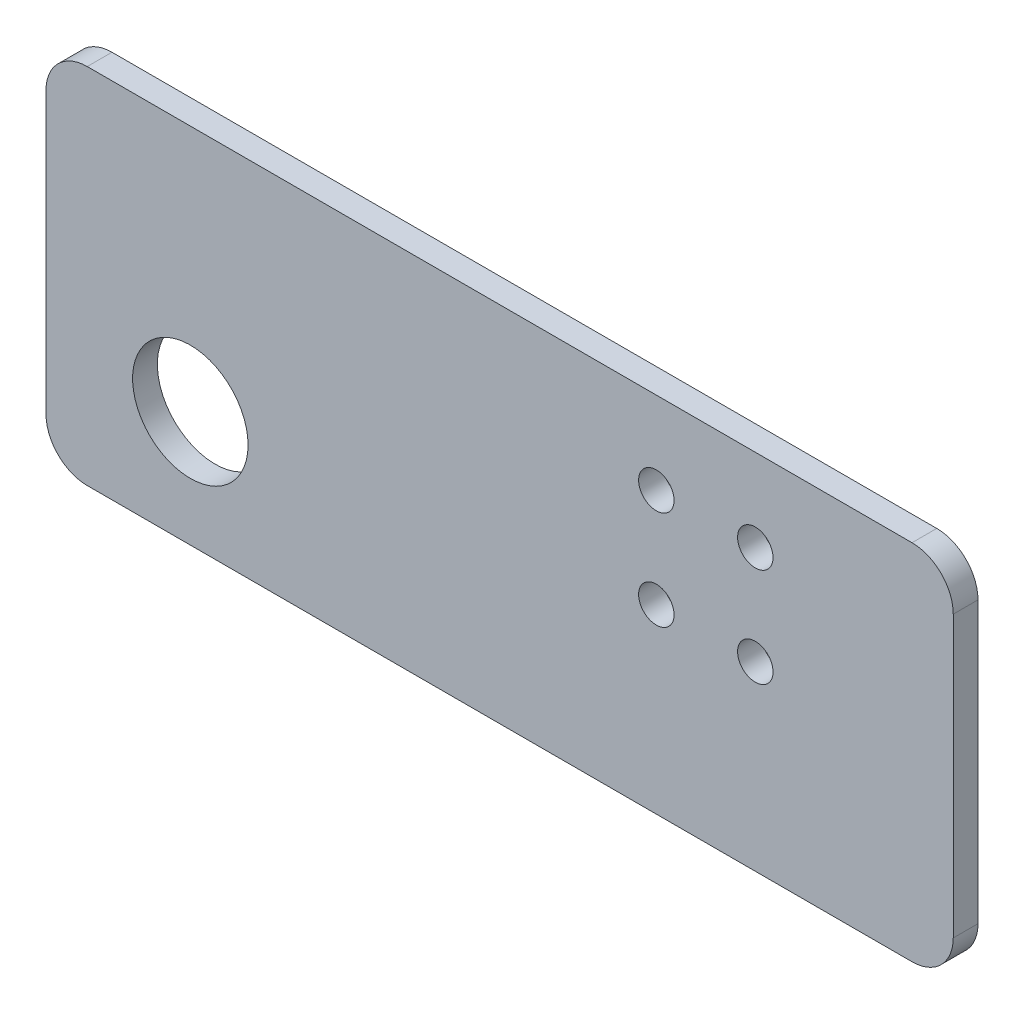
SolidWorks part; units mm, degrees
ref_plane "前视基准面" through (0, 0, 0) normal (0, 0, 1) x (1, 0, 0)
ref_plane "上视基准面" through (0, 0, 0) normal (0, 1, 0) x (1, 0, 0)
ref_plane "右视基准面" through (0, 0, 0) normal (1, 0, 0) x (0, 0, -1)
sketch "草图1" plane through (0, 0, 0) normal (0, 0, 1) x (1, 0, 0)
  line L1 (-80, 22) -> (80, 22)
  line L2 (-80, 22) -> (-80, -22)
  line L3 (-80, -22) -> (80, -22)
  line L4 (80, 22) -> (80, -22)
  line L5 (-80, 22) -> (80, -22) construction
  line L6 (-80, -22) -> (80, 22) construction
  point P0 (0, 0)
  dimension "D1" = 160
  dimension "D2" = 44
extrude "凸台-拉伸1" add sketch "草图1" along normal blind 3
sketch "草图2" plane through (0, 0, 3) normal (0, 0, 1) x (1, 0, 0)
  line L0 (-62.5, -8) -> (0, -8) construction
  line L1 (0, -8) -> (62.5, -8) construction
  line L3 (-6, 12) -> (6, 12) construction
  line L4 (-6, 12) -> (-6, 0) construction
  line L5 (-6, 0) -> (6, 0) construction
  line L6 (6, 12) -> (6, 0) construction
  line L7 (-6, 12) -> (6, 0) construction
  line L8 (-6, 0) -> (6, 12) construction
  line L10 (80, 22) -> (-80, 22) construction
  line L11 (0, -8) -> (0, -22) construction
  line L12 (-80, -22) -> (80, -22) construction
  circle A0 centre (-62.5, -8) radius 7
  circle A1 centre (62.5, -8) radius 7
  circle A2 centre (-6, 12) radius 2.15
  circle A3 centre (6, 12) radius 2.15
  circle A4 centre (6, 0) radius 2.15
  circle A5 centre (-6, 0) radius 2.15
  dimension "D2" = 14
  dimension "D4" = 4.3
  dimension "D1" = 125
  dimension "D3" = 12
  dimension "D5" = 10
  dimension "D6" = 14
extrude "切除-拉伸1" cut sketch "草图2" against normal blind 3
fillet "圆角1" radius 5 4 edges at (80, 22, 1.5) (80, -22, 1.5) (-80, 22, 1.5) (-80, -22, 1.5)
sketch "草图3" plane through (0, 0, 3) normal (0, 0, 1) x (1, 0, 0)
  line L0 (80, -17) -> (80, 17) construction
  line L1 (93.6784, -36.1637) -> (30, -36.1637)
  line L2 (93.6784, -36.1637) -> (93.6784, 36.3489)
  line L3 (93.6784, 36.3489) -> (30, 36.3489)
  line L4 (30, -36.1637) -> (30, 36.3489)
  dimension "D1" = 50
extrude "切除-拉伸2" cut sketch "草图3" against normal blind 10
fillet "圆角2" radius 5 2 edges at (30, -22, 1.5) (30, 22, 1.5)
